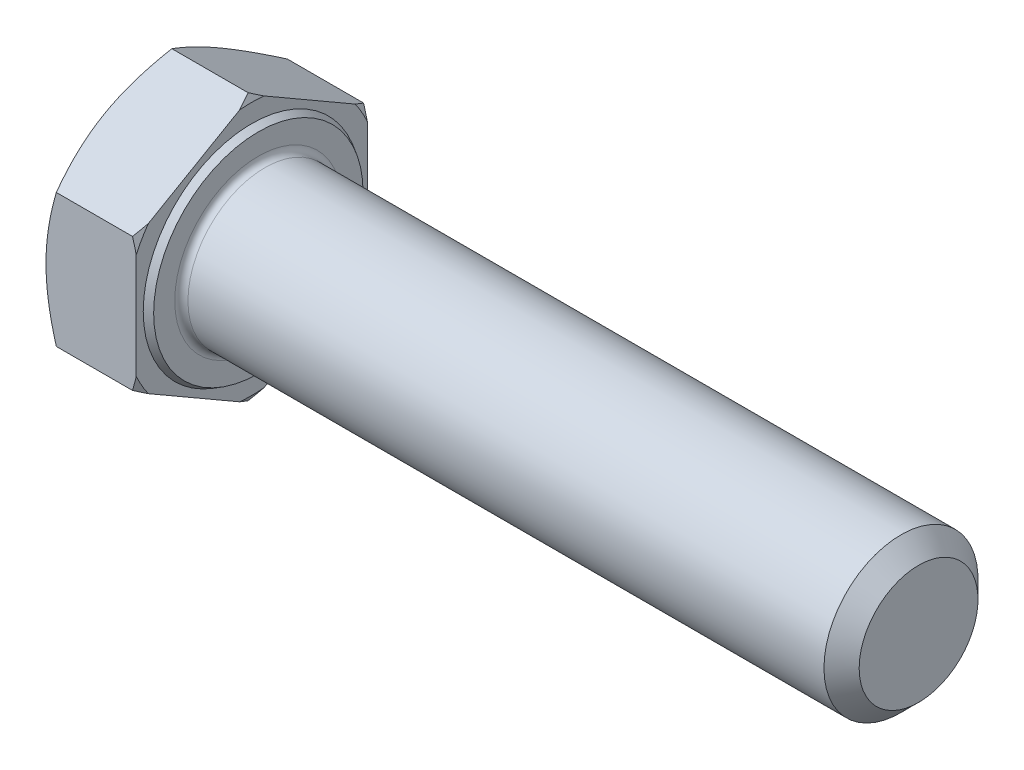
SolidWorks part; units mm, degrees
material "Steel"
ref_plane "Front" through (0, 0, 0) normal (0, 0, 1) x (1, 0, 0)
ref_plane "Top" through (0, 0, 0) normal (0, 1, 0) x (1, 0, 0)
ref_plane "Right" through (0, 0, 0) normal (1, 0, 0) x (0, 0, -1)
sketch "Dimension Sketch" plane through (0, 0, 0) normal (0, 0, 1) x (1, 0, 0)
  line L0 (0, 0) -> (34, 0) construction
  line L1 (0, 0) -> (0, 14) construction
  point P3 (2, 0)
  point P4 (0.6, 0)
  point P6 (0, 16.7)
  point P7 (0, 14.7)
  point P8 (0, 19.15)
  point P9 (22.78, 0)
  point P10 (8.8, 0)
  point P11 (5.85, 0)
  point P12 (0.6, 0)
  point P13 (21, 0)
  point P14 (60, 0)
  point P15 (26, 0)
  point P16 (50, 0)
  dimension "b(参考)" = 34
  dimension "P" = 2
  dimension "d" = 14
  dimension "c(max)" = 0.6
  dimension "da(max)" = 16.7
  dimension "ds(max)" = 14.7
  dimension "dw(min)" = 19.15
  dimension "e(min)" = 22.78
  dimension "k(公称)" = 8.8
  dimension "kw(min)" = 5.85
  dimension "r(min)" = 0.6
  dimension "s(公称)" = 21
  dimension "l" = 60
  dimension "lg(max)" = 26
  dimension "ls(min)" = 16
sketch "Sketch1" plane through (0, 0, 0) normal (1, 0, 0) x (0, 0, -1)
  line L0 (10.5, 6.0622) -> (10.5, -6.0622)
  line L1 (-10.5, 6.0622) -> (-10.5, -6.0622)
  line L2 (10.5, -6.0622) -> (0, -12.1244)
  line L3 (0, -12.1244) -> (-10.5, -6.0622)
  line L4 (10.5, 6.0622) -> (0, 12.1244)
  line L5 (0, 12.1244) -> (-10.5, 6.0622)
  point P6 (0, 10.6556)
  dimension "D1" = 22.78
  dimension "s" = 21
  dimension "D2" = 120
  dimension "D3" = 10.5
  dimension "D4" = 10.5
  dimension "D5" = 10.5
extrude "Boss-Extrude" add sketch "Sketch1" along normal blind 8.8
sketch "Sketch2" plane through (0, 0, 0) normal (0, 0, 1) x (1, 0, 0)
  line L0 (0, 6.0622) -> (0, -6.0622) construction
  line L1 (0, 0) -> (68.8, 0)
  line L2 (0, 0) -> (0, 7)
  line L3 (0, 7) -> (8.8, 7)
  line L4 (68.8, 0) -> (68.8, 5.268)
  line L5 (8.8, 12.1244) -> (8.8, 6.0622) construction
  line L7 (0, 0) -> (-51.1435, 0) construction
  line L8 (68.8, -5.268) -> (8.8, -7) construction
  line L9 (0, -7) -> (8.8, -7) construction
  line L10 (10.8, 7) -> (10.8, 0) construction
  line L11 (34.8, 7) -> (34.8, 0) construction
  line L12 (8.8, 6.0622) -> (8.8, -6.0622) construction
  line L13 (8.8, 7) -> (68.8, 7)
  line L14 (68.8, 7) -> (68.8, 5.268)
  dimension "l" = 60
  dimension "d" = 14
  dimension "Minor_dia" = 10.536
  dimension "p" = 2
  dimension "b" = 34
revolve "Boss-Revolve1" add sketch "Sketch2" angle 360 about L7
cosmetic thread "Cosmetic Thread1" parameters "D1"=34, "D2"=11.2
sketch "Sketch3" plane through (0, 0, 0) normal (0, 0, 1) x (1, 0, 0)
  line L0 (0, 10.5) -> (3.8246, 17.1244)
  line L1 (0, 12.1244) -> (0, 6.0622) construction
  line L2 (3.8246, 17.1244) -> (3.8246, 22.1244)
  line L3 (3.8246, 22.1244) -> (-10, 22.1244)
  line L4 (-10, 22.1244) -> (-10, 10.5)
  line L5 (-10, 10.5) -> (0, 10.5)
  line L6 (0, 0) -> (99.06, 0) construction
  line L7 (8.8, 12.1244) -> (0, 12.1244) construction
  dimension "D1" = 10.5
  dimension "D2" = 5
  dimension "D3" = 10
  dimension "D4" = 5
  dimension "Head_ch_ang" = 30
revolve "Cut-Revolve1" cut sketch "Sketch3" angle 360 about L6
sketch "Sketch5" plane through (0, 0, 0) normal (0, 0, 1) x (1, 0, 0)
  line L0 (8.8, 10.5) -> (4.9754, 17.1244)
  line L1 (8.8, 12.1244) -> (8.8, 6.0622) construction
  line L2 (4.9754, 17.1244) -> (4.9754, 22.1244)
  line L3 (4.9754, 22.1244) -> (14.9754, 22.1244)
  line L4 (14.9754, 22.1244) -> (14.9754, 10.5)
  line L5 (14.9754, 10.5) -> (8.8, 10.5)
  line L7 (8.8, 12.1244) -> (0.9378, 12.1244) construction
  line L8 (0, 0) -> (99.06, 0) construction
  line L9 (0, 0) -> (99.06, 0) construction
  dimension "D1" = 10.5
  dimension "D2" = 5
  dimension "D3" = 10
  dimension "Head_ch_ang" = 30
  dimension "D4" = 5
revolve "Cut-Revolve2" cut sketch "Sketch5" angle 360 about L8
sketch "Sketch4" plane through (0, 0, 0) normal (0, 0, 1) x (1, 0, 0)
  line L0 (8.7, 9.575) -> (8.7, 0) construction
  line L1 (8.8, 12.1244) -> (8.8, 6.0622) construction
  line L2 (8.8, 9.5173) -> (8.2, 9.8637)
  line L3 (8.8, 9.5173) -> (8.8, 22.1244)
  line L4 (8.8, 22.1244) -> (8.2, 22.1244)
  line L5 (0, 0) -> (95.25, 0) construction
  line L6 (-51.1435, 0) -> (0, 0) construction
  line L7 (8.2, 9.8637) -> (8.2, 22.1244)
  line L8 (7.8622, 12.1244) -> (0.9378, 12.1244) construction
  line L9 (8.8, 9.0933) -> (8.8, 10.5) construction
  line L10 (7.8622, 12.1244) -> (0.9378, 12.1244) construction
  point P15 (2.85, 12.1244)
  dimension "D1" = 120
  dimension "D2" = 10
  dimension "D3" = 0.1
  dimension "c" = 0.6
  dimension "D4" = 19.15
  dimension "D5" = 5.85
revolve "Cut-Revolve3" cut sketch "Sketch4" angle 360 about L5
chamfer "Chamfer" distance 1.6 angle 45 1 edges at (68.8, 0, -7)
sketch "Sketch9" plane through (0, 0, 0) normal (0, 0, 1) x (1, 0, 0)
  line L0 (8.8, -9.5173) -> (8.8, 9.5173) construction
  line L1 (67.2, 7) -> (8.8, 7) construction
  line L2 (0, 0) -> (8.8, 0) construction
  line L3 (8.8, 7.6) -> (8.8, 7)
  line L4 (8.8, 7) -> (9.4, 7)
  arc A0 (8.8, 7.6) -> (9.4, 7) centre (9.4, 7.6) ccw
  dimension "D1" = 0.6
revolve "Revolve1" add sketch "Sketch9" angle 360 about L2
sketch "Sketch6" plane through (0, 0, 0) normal (0, 0, 1) x (1, 0, 0)
  line L0 (66.2, -5.268) -> (65.2001, -7)
  line L1 (66.2, -5.268) -> (67.2, -7)
  line L2 (67.2, -7) -> (67.2, -12.1244)
  line L3 (-3.175, 0) -> (0, 0) construction
  line L4 (67.2, -7) -> (67.2, 7) construction
  line L5 (67.2, -12.1244) -> (65.2001, -12.1244)
  line L6 (65.2001, -12.1244) -> (65.2001, -7)
  line L7 (9.4, -7) -> (67.2, -7) construction
  line L9 (7.8622, -12.1244) -> (0.9378, -12.1244) construction
  dimension "Thread_minor" = 10.536
  dimension "SideAngle" = 60
  dimension "VeeAngle" = 60
revolve "Cut-Revolve4" [suppressed] cut sketch "Sketch6" angle 360 about L3
pattern_linear "LPattern1" [suppressed]
